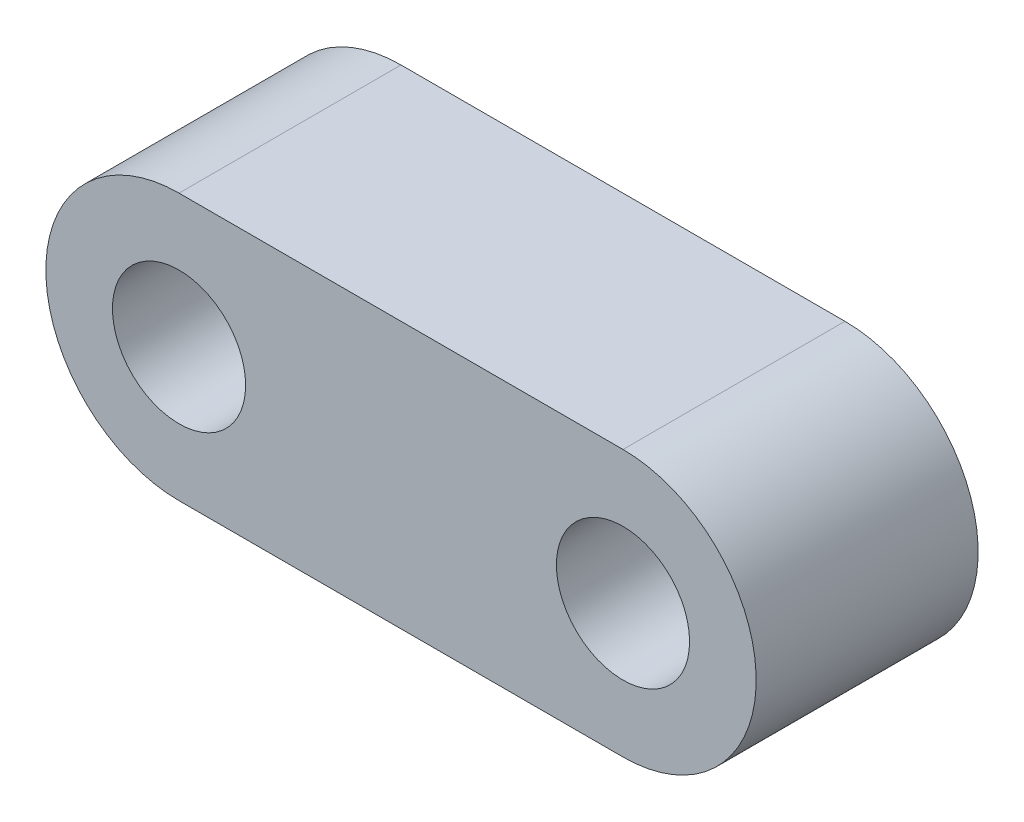
from build123d import *

# Parameters (mm, degrees)
SKETCH1_R           = 3
BOSS_EXTRUDE1_DEPTH = 10


with BuildPart() as part:
    # Sketch1 → Boss-Extrude1 (new body)
    with BuildSketch(Plane.XY):
        with BuildLine():
            Line((0, -6), (20, -6))
            ThreePointArc((20, -6), (26, 0), (20, 6))
            Line((20, 6), (0, 6))
            ThreePointArc((0, 6), (-6, 0), (0, -6))
        make_face()
        Circle(SKETCH1_R, mode=Mode.SUBTRACT)
        with Locations((20, 0)):
            Circle(SKETCH1_R, mode=Mode.SUBTRACT)
    extrude(amount=BOSS_EXTRUDE1_DEPTH)


solid = part.part
